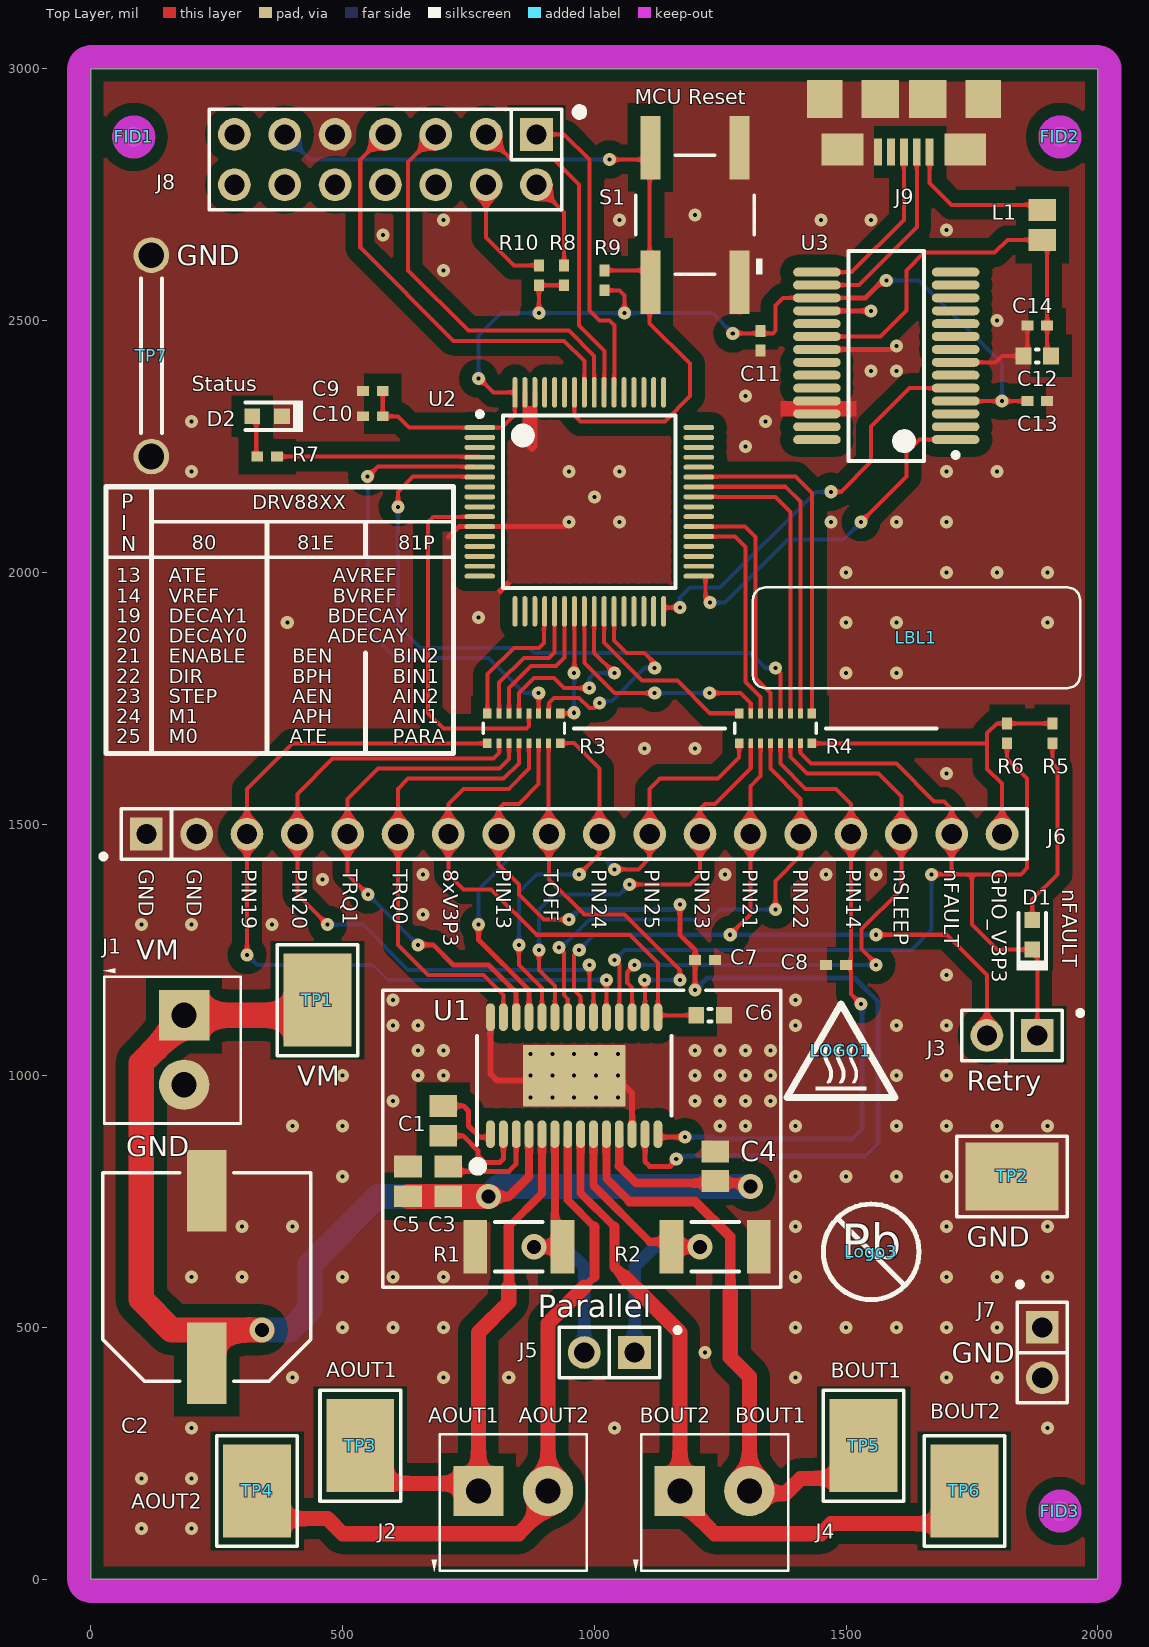
[diagram p0: Top Layer view]
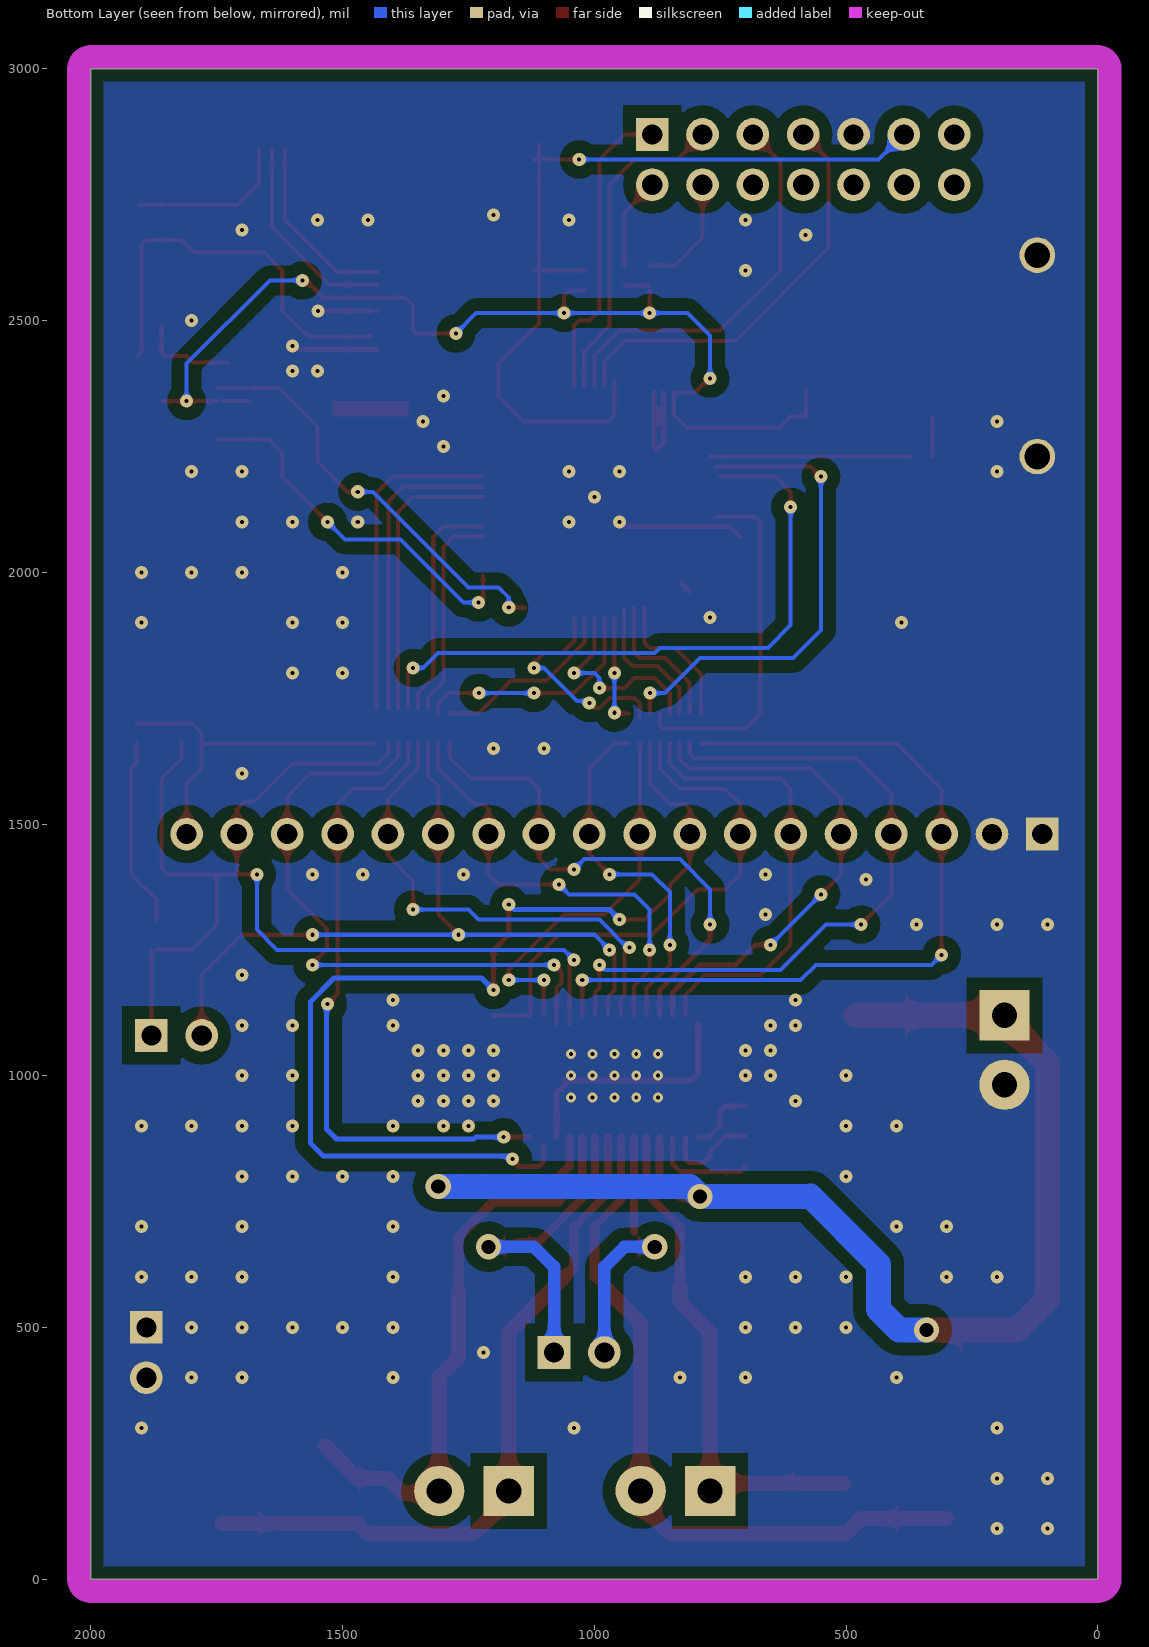
[diagram p1: Bottom Layer view, seen from below]
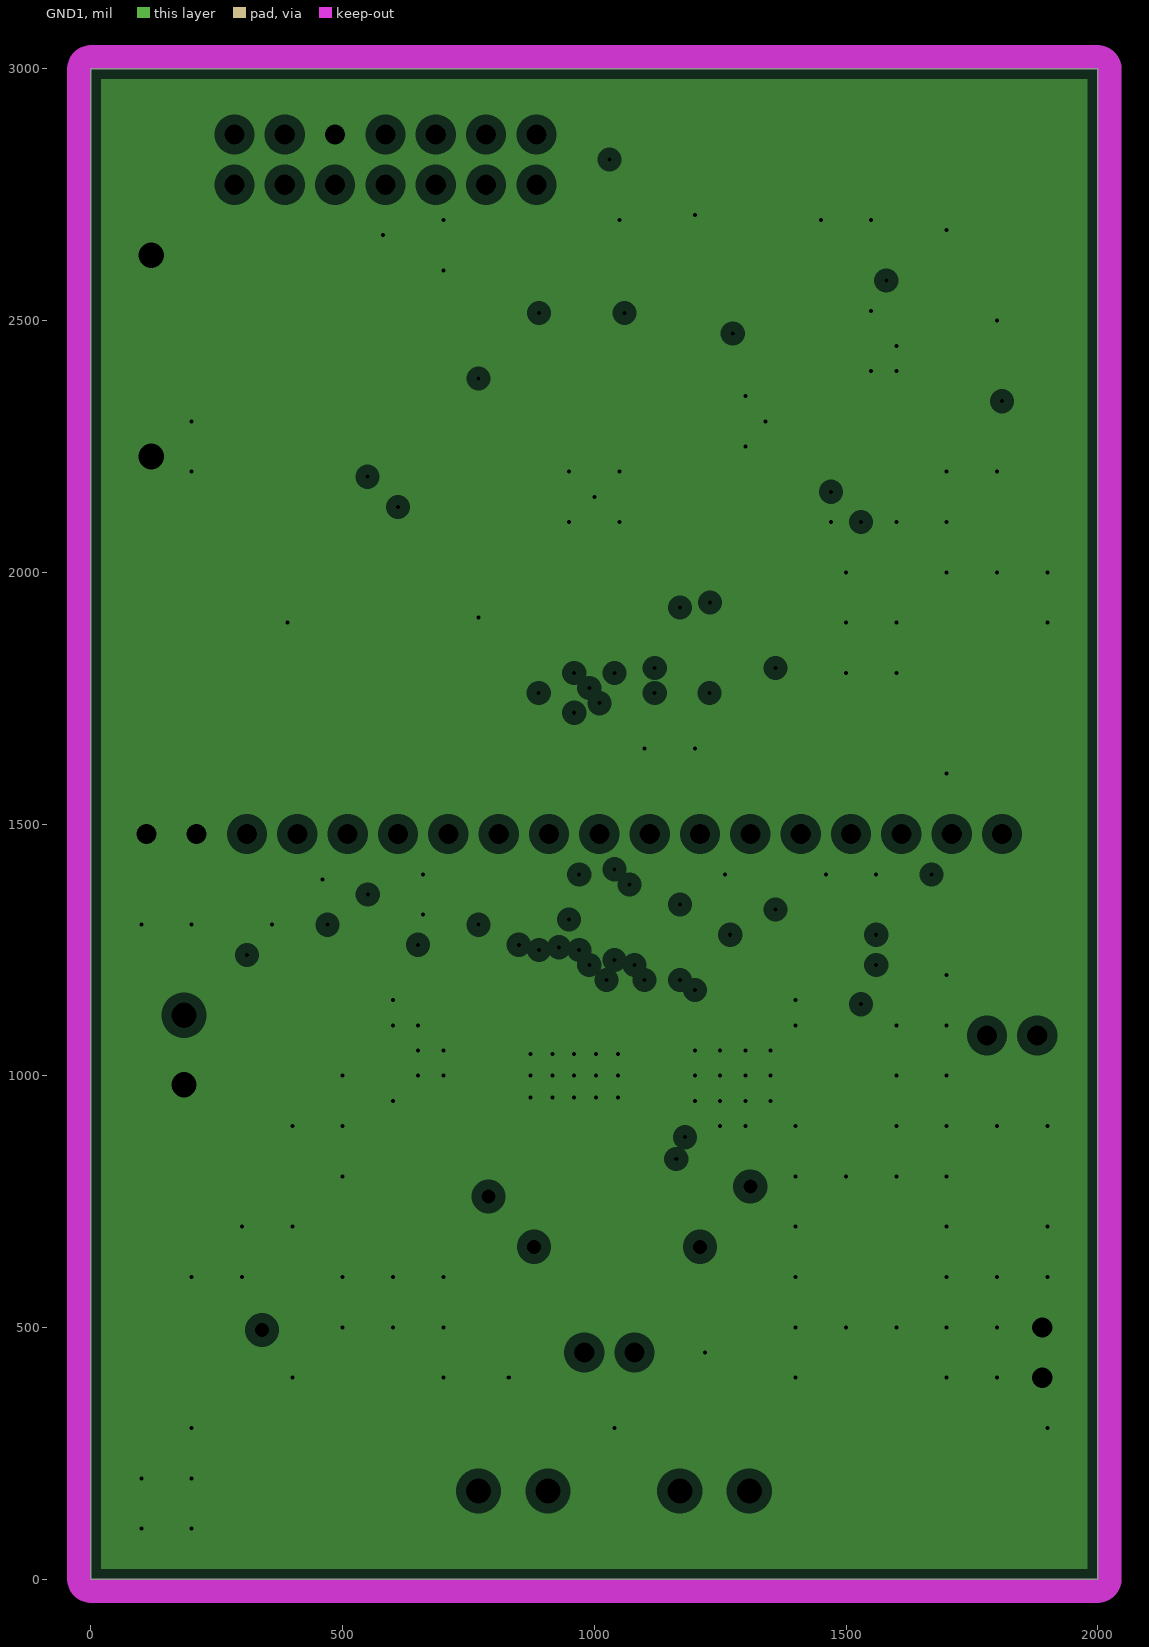
[diagram p2: GND1, clearances drawn from the general rule]
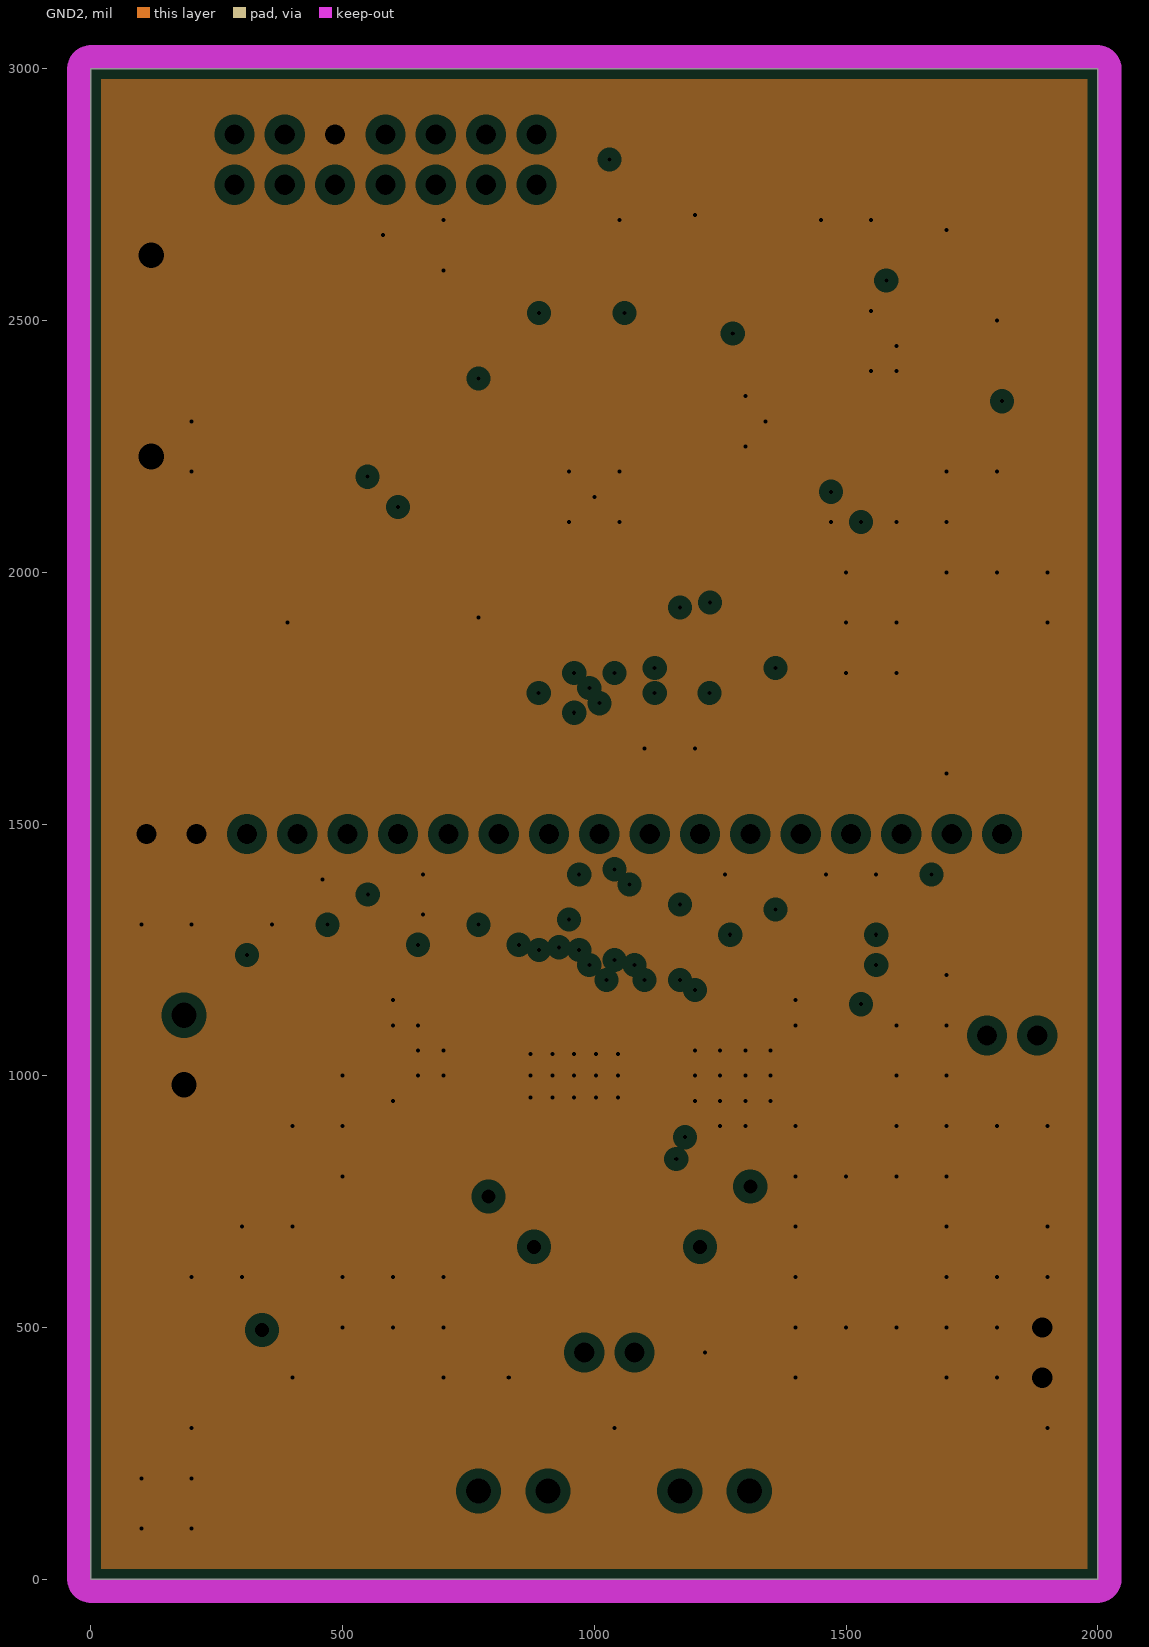
[diagram p3: GND2, clearances drawn from the general rule]
# Altium PCB MISC86176.PcbDoc (part 1 of 2)
Units mil, origin at the board's own origin, x right, y up, seen from the top; angles counter-clockwise.
Board outline 2000 x 3000 mil, 4 copper layers (Top Layer, GND1, GND2, Bottom Layer), stack 91.4 mil thick; 53 components, 60 nets, 274 pads, 201 vias.

## Layer stack, top to bottom
Top Layer: signal copper 2.1
Dielectric: core 59.2, FR-4, Dk 4.8
GND1: plane copper 1.4, net GND
Dielectric: prepreg 12.6, FR-4, Dk 4.8
GND2: plane copper 1.4, net GND
Dielectric: core 12.6, FR-4, Dk 4.8
Bottom Layer: signal copper 2.1

## Board outline
0,0 0,3000 2000,3000 2000,0

## Design rules (kind name [scope] priority, off if disabled: settings)
AcuteAngle [All] p1: minimum=4.50000000000000E+0001
Clearance Clearance_Keepouts [((IsTrack Or IsArc) And Not InPoly) And IsFree and IsKeepOut vs ((IsTrack Or IsArc) And Not InPoly) And IsFree and IsKeepOut] p1: gap=0
Clearance Clearance_BoardEdge_MountingHoles [OnCopper and InComponentClass('Mounting Holes') vs IsKeepOut] p2: gap=40
Clearance Clearance_BoardEdge_Poly [OnCopper and InPoly vs IsKeepOut] p3: gap=25
Clearance Clearance_BoardEdge [OnCopper and Not InComponentClass('Logo') and not InComponentClass('FiducialMark') and not InRegion(1000,500,4000,800) and Not IsKeepout vs IsKeepOut] p4: gap=20
Clearance Clearance_Poly [InPolygon] p5: gap=25
Clearance [All] p6: gap=7.87
ComponentClearance ComponentClearance_MountingHoles_FiducialMarks [InComponentClass('Mounting Holes') vs InComponentClass('FiducialMark')] p1: gap=50 collisioncheckmode=3 verticalgap=10 showdistances=FALSE
ComponentClearance ComponentClearance_Shunt [InComponentClass('Header') vs InComponentClass('Shunt')] p2: gap=0 collisioncheckmode=3 verticalgap=0 showdistances=FALSE
ComponentClearance ComponentClearance_Logo [InComponentClass('Logo')] p3: gap=50 collisioncheckmode=3 verticalgap=10 showdistances=FALSE
ComponentClearance ComponentClearance_ScrewToNut [(HasFootprint('NY PMS 440 0025 PH')) vs (HasFootprint('Keystone_1902C'))] p4: gap=5 collisioncheckmode=3 verticalgap=10 showdistances=FALSE
ComponentClearance ComponentClearance_MountingHoles [InComponentClass('Mounting Holes')] p5: gap=250 collisioncheckmode=3 verticalgap=100000 showdistances=FALSE
ComponentClearance ComponentClearance_SmallPassives [HasFootprint('0201*') or HasFootprint('0402*') or HasFootprint('0508') or HasFootprint('0603*') or HasFootprint('0612') or HasFootprint('0805*') or HasFootprint('0815*') or HasFootprint('0830*') or HasFootprint('1206*') or HasFootprint('1210*') or HasFootprint('1808*') or HasFootprint('1812*') or HasFootprint('1825*') or HasFootprint('2010*') or HasFootprint('2220*') or HasFootprint('2225*') or HasFootprint('2512*') or HasFootprint('2728*') or HasFootprint('3518*') vs HasFootprint('0201*') or HasFootprint('0402*') or HasFootprint('0508') or HasFootprint('0603*') or HasFootprint('0612') or HasFootprint('0805*') or HasFootprint('0815*') or HasFootprint('0830*') or HasFootprint('1206*') or HasFootprint('1210*') or HasFootprint('1808*') or HasFootprint('1812*') or HasFootprint('1825*') or HasFootprint('2010*') or HasFootprint('2220*') or HasFootprint('2225*') or HasFootprint('2512*') or HasFootprint('2728*') or HasFootprint('3518*')] p6: gap=20 collisioncheckmode=3 verticalgap=10 showdistances=FALSE
ComponentClearance ComponentClearance_THtoSMT [IsThruComponent vs IsSMTComponent] p7: gap=100 collisioncheckmode=3 verticalgap=30 showdistances=FALSE
ComponentClearance ComponentClearance_THtoTH [IsThruComponent vs IsThruComponent] p8: gap=118.11 collisioncheckmode=3 verticalgap=30 showdistances=FALSE
ComponentClearance [All] p9: gap=40 collisioncheckmode=3 verticalgap=10 showdistances=FALSE
DiffPairsRouting [All] p1: maxlimit=100 minlimit=10 mostfreqgap=10 maxuncoupledlength=1000
FabricationTestPointUsage TestPointUsage [All] p1: valid=2 allowmultiple=FALSE
FabricationTestpoint Testpoint [(IsPad And (OnTopLayer Or OnBottomLayer))] p1: side=3 testpointundercomponent=TRUE minsize=40 maxsize=100 preferedsize=60 minholesize=0 maxholesize=40 preferedholesize=32 testpointgrid=1 allowsidetop=TRUE allowsidebottom=TRUE usegrid=TRUE gridtolerance=0.01
FanoutControl Fanout_LCC [IsLCC] p1: bgadir=Out bgaviamode=Centered fanoutstyle=Auto fanoutdirection=Alternating viagrid=1 // Fanout_LCC (Default Rule)
FanoutControl Fanout_BGA [IsBGA] p2: bgadir=Out bgaviamode=Centered fanoutstyle=Auto fanoutdirection=Alternating viagrid=1 // Fanout_BGA (Default Rule)
FanoutControl Fanout_Default [All] p4: bgadir=Out bgaviamode=Centered fanoutstyle=Auto fanoutdirection=Alternating viagrid=1 // Fanout_Default (Default Rule)
FanoutControl Fanout_Small [(CompPinCount < 5)] p5: bgadir=Out bgaviamode=Centered fanoutstyle=Auto fanoutdirection=OutThenIn viagrid=1 // Fanout_Small (Default Rule)
HoleSize [All] p1: absolutevalues=TRUE maxlimit=251 minlimit=7.87 maxpercent=80.000 minpercent=20.000
MinimumAnnularRing MinimumAnnularRing_ThermalPadVias [IsVia and InAnyComponent] p1: minimumring=3.94
MinimumAnnularRing [All] p2: minimumring=5
MinimumSolderMaskSliver MinimumSolderMaskSliver_Logo [InComponentClass('Logo') vs InComponentClass('Logo')] p1: minsoldermaskwidth=0.7
MinimumSolderMaskSliver [All] p2: minsoldermaskwidth=3.94
PlaneClearance [All] p1: clearance=20
PlaneConnect [All] p1: planeconnectstyle=Relief reliefexpansion=10 reliefentries=4 reliefconductorwidth=10 reliefairgap=10
PolygonConnect PolygonConnect_2 [All vs IsNamedPolygon('Top Layer-GND')] p1: connectstyle=Direct reliefconductorwidth=10 reliefentries=4 polygonreliefangle="90 Angle"
PolygonConnect PolygonConnect_1 [All vs IsNamedPolygon('Bottom Layer-GND')] p2: connectstyle=Direct reliefconductorwidth=10 reliefentries=4 polygonreliefangle="90 Angle"
PolygonConnect [All] p3: connectstyle=Relief reliefconductorwidth=10 reliefentries=4 polygonreliefangle="90 Angle"
RoutingVias ThermalPadVias [IsVia and InAnyComponent] p1: holewidth=7.87 width=19.68 viastyle="Through Hole" minholewidth=7.87 minwidth=15.75 maxholewidth=12.99 maxwidth=23.62
RoutingVias [All] p2: holewidth=16 width=34 viastyle="Through Hole" minholewidth=7.87 minwidth=26 maxholewidth=40 maxwidth=65
SilkToSilkClearance SilkToSilkClearance_Pb-FreeLogo [(HasFootprint('Pb-Free_Overlay_Medium') OR HasFootprint('Pb-Free_Overlay_Small')) vs (HasFootprint('Pb-Free_Overlay_Medium') OR HasFootprint('Pb-Free_Overlay_Small'))] p1: silktosilkclearance=0
SilkToSilkClearance [All] p2: silktosilkclearance=3
SilkscreenOverComponentPads "Silk to Solder Mask Opening" [All] p1: minsilkscreentomaskgap=3
SolderMaskExpansion [All] p1: expansion=1.97
Width [All] p1: maxlimit=100 minlimit=6 preferedwidth=10 checkconnectedcopper=TRUE
14 further rules are at their usual default settings.

## Classes and differential pairs
component class Header: J3 J5 J6 J7 J8
component class MDBU004A_DRV888x: C1 C2 C3 C4 C5 C6 C7 C8 D1 J1 J2 J3 J4 J5 J6 J7 R1 R2 R3 R4 R5 R6 TP1 TP2 TP3 TP4 TP5 TP6 TP7 U1
component class MDBU004A_DRV888x_MSP430F2617: C9 C10 C11 C12 C13 C14 D2 J8 J9 L1 R7 R8 R9 R10 S1 U2 U3
component class Logo: Logo2
component class MDBU004A_Hardware: FID1 FID2 FID3 LBL1 LOGO1 Logo2 Logo3 Logo4 ZZ1 ZZ2 ZZ3 ZZ4 ZZ5
component class FiducialMark: FID1 FID2 FID3
component class AssemblyNote: ZZ1 ZZ2 ZZ3 ZZ4 ZZ5
component class Label: LBL1

## Components (designator, comment, footprint, x,y, rotation, side; value= is the part's Value field where it differs from the comment)
C1 "C0805C104K1RACTU" 0805L 700,910 r270 top
C2 "EEE-FK1J101P" SM_RADIAL_G 230,600 r90 top
C3 "C2012X7R1E474K" 0805L 710,790 r270 top
C4 "C0805C104K1RACTU" 0805L 1240,820 r270 top
C5 "C0805C104K1RACTU" 0805L 630,790 r270 top
C6 "C0603C474K9RACTU" 0603L 1230,1120 r0 top
C7 "GRM155R61A104KA01D" 0402L 1220,1230 r0 top
C8 "GRM155R61A104KA01D" 0402L 1480,1220 r180 top
C9 "GRM155R61A104KA01D" 0402L 560,2360 r180 top
C10 "GRM155R61A104KA01D" 0402L 560,2310 r180 top
C11 "GRM155R61A104KA01D" 0402L 1330,2460 r270 top
C12 "CGB3B1X5R1A475K055AC" 0603L 1880,2430 r180 top
C13 "GRM155R61A105KE15D" 0402L 1880,2340 r0 top
C14 "GRM155R61A104KA01D" 0402L 1880,2490 r180 top
D1 "LTST-C190CKT" LED_LTST-C190_Red 1870,1280 r270 top
D2 "LTST-C190GKT" LED_LTST-C190 350,2310 r0 top
FID1 "Fiducial" Fiducial10-20 85,2865 r90 top
FID2 "Fiducial" Fiducial10-20 1925,2865 r90 top
FID3 "Fiducial" Fiducial10-20 1925,135 r90 top
J1 "ED555/2DS" TERM_BLK_ED555-2DS 185,1120 r270 top
J2 "ED555/2DS" TERM_BLK_ED555-2DS 770,175 r0 top
J3 "90120-0122" CONN_90120-0122 1830,1080 r180 top
J4 "ED555/2DS" TERM_BLK_ED555-2DS 1170,175 r0 top
J5 "90120-0122" CONN_90120-0122 1030,450 r180 top
J6 "TSW-118-07-G-S" TSW-118-07-G-S 960,1480 r0 top
J7 "90120-0122" CONN_90120-0122 1890,450 r270 top
J8 "PEC07DAAN" CONN_PEC07DAAN 585,2820 r180 top
J9 "ZX62-B-5PA(11)" CONN_USB_micro_ZX62-B-5PA 1615,2835 r180 top
L1 "MMZ2012R300A" 0805L 1890,2690 r90 top
LBL1 "Size: 0.65\" x 0.20 \"" Label_650x200 1640,1870 r0 top
LOGO1 "CAUTION HOT SURFACE" IEC_HotSurface_Small 1490,1050 r0 top
Logo3 "Pb-Free Symbol" Pb-Free_Overlay_Medium 1550,650 r0 top
R1 "CSRN2010FKR250" 2010L 850,660 r0 top
R2 "CSRN2010FKR250" 2010L 1240,660 r180 top
R3 "EXB-2HV330JV" RESCAXS_EXB-2HV 860,1690 r0 top
R4 "EXB-2HV330JV" RESCAXS_EXB-2HV 1360,1690 r0 top
R5 "CRCW0402510RJNED" 0402L 1910,1680 r90 top
R6 "CRCW04024K99FKED" 0402L 1820,1680 r90 top
R7 "CRCW0402330RJNED" 0402L 350,2230 r0 top
R8 "ERJ-2GE0R00X" 0402L 940,2590 r90 top
R9 "CRCW04023K32FKED" 0402L 1020,2580 r270 top
R10 "ERJ-2GE0R00X" 0402L 890,2590 r90 top
S1 "EVQP1D05M" SW_EVQxxx05M 1200,2710 r180 top
TP1 "5016" Testpoint_Keystone_Compact 450,1150 r90 top
TP2 "5016" Testpoint_Keystone_Compact 1830,800 r180 top
TP3 "5016" Testpoint_Keystone_Compact 535,265 r90 top
TP4 "5016" Testpoint_Keystone_Compact 330,175 r90 top
TP5 "5016" Testpoint_Keystone_Compact 1535,265 r90 top
TP6 "5016" Testpoint_Keystone_Compact 1735,175 r90 top
TP7 "D3082-05" Harwin_D3082-05 120,2430 r270 top
U1 "DRV8880PWPR" PWP0028C_N 960,1000 r90 top
U2 "MSP430F2617TPM" PM0064A_L 990,2140 r0 top
U3 "FT232RL" SSOP28_M 1580,2430 r180 top

## Footprints (in the part's own frame and the unit in brackets; to place one, negate y for a bottom-side part, rotate by r counter-clockwise, add the part's x,y. Pads: shape width x height; smd on the part's side, far side on the other; paste and mask are expansions set on the pad)
0402L [mm] "0402 from SM-752 data"
  rect 0.6x0.5 smd: 1(-0.5,0) 2(0.5,0)
  body extent -0.55,-0.3 0.55,0.3, height 0.6
0603L [mm] "0603 from SM-752 data"
  rect 0.8x0.85 smd: 1(-0.7,0) 2(0.7,0)
  silkscreen extent -0.07,-0.33 0.07,0.33, body extent -0.87,-0.47 0.87,0.47, height 0.85
0805L [mm] "0805 from SM-752 data"
  rect 1.1x1.4 smd: 1(-0.75,0) 2(0.75,0)
  body extent -1.1,-0.72 1.1,0.72, height 1.1
2010L [mm]
  rect 1.2x2.7 smd: 1(-2.2,0) 2(2.2,0)
  silkscreen extent -1.2,-1.25 1.2,1.25, body extent -2.73,-1.45 2.73,1.45, height 1.66
CONN_90120-0122 [mm] "Molex"
  rect 1.65x1.65 hole 1.016 mask+0: 1(-1.27,0)
  round 1.65 hole 1.016 mask+0: 2(1.27,0)
  silkscreen extent -3.57,-1.27 2.54,1.27, body extent -2.54,-1.27 2.54,1.27, height 9.29
CONN_PEC07DAAN [mm] "SULLINS"
  rect 1.65x1.65 hole 1.016 mask+0: 1(-7.62,-1.27)
  round 1.65 hole 1.016 mask+0: 2(-7.62,1.27) 3(-5.08,-1.27) 4(-5.08,1.27) 5(-2.54,-1.27) 6(-2.54,1.27) 7(0,-1.27) 8(0,1.27) 9(2.54,-1.27) 10(2.54,1.27) 11(5.08,-1.27) 12(5.08,1.27) 13(7.62,-1.27) 14(7.62,1.27)
  silkscreen extent -9.99,-2.6 8.89,2.54, body extent -8.95,-2.6 8.95,2.6, height 11.43
CONN_USB_micro_ZX62-B-5PA [mm] "Hirose"
  rect 0.4x1.35 smd: 1(-1.3,0) 2(-0.65,0) 3(0,0) 4(0.65,0) 5(1.3,0)
  rect 1.9x1.9 smd: 6(-1.2,-2.675) 7(1.2,-2.675)
  rect 1.8x1.9 smd: 8(-4,-2.675) 9(4,-2.675)
  rect 2.1x1.6 smd: 10(-3.1,-0.125) 11(3.1,-0.125)
  body extent -3.75,-5.32 3.75,0.18, height 2.55
Fiducial10-20 [mm]
  round 1 smd mask+0.5: 1(0,0)
  Top Layer keep-out circle w1.178: c0,0 r0.5
Harwin_D3082-05 [mm] "Shorting Plug, 10.16mm spacing, TH"
  round 1.8 hole 1.3: 1(-5.08,0) 2(5.08,0)
  silkscreen extent -3.9,-0.53 3.9,0.53, body extent -5.6,-0.52 5.61,0.52, height 6.63
IEC_HotSurface_Small [mil]
  silkscreen extent -107,-93 107,92
Label_650x200 [mil] "Thermal Transfer Label"
  round 1 on Mech13: 0(0,0)
  silkscreen extent -325,-100 325,100, body extent -326,-101 326,101, height 1
LED_LTST-C190 [mm] "Lite-On"
  rect 0.8x0.8 smd: 1(-0.75,0) 2(0.75,0)
  silkscreen extent -1.1,-0.8 1.8,0.8, body extent -0.85,-0.45 0.85,0.45, height 0.9
LED_LTST-C190_Red [mm] "Lite-On"
  rect 0.8x0.8 smd: 1(-0.75,0) 2(0.75,0)
  silkscreen extent -1.1,-0.8 1.8,0.8, body extent -0.85,-0.45 0.85,0.45, height 0.9
Pb-Free_Overlay_Medium [mil]
  silkscreen extent -95,-95 95,95
PM0064A_L [mm] "Thin QFP, 64-Leads, Body 10x10mm, Pitch 0.5mm, IPC High Density"
  oval 1.55x0.25 smd: 1(-5.525,3.75) 2(-5.525,3.25) 3(-5.525,2.75) 4(-5.525,2.25) 5(-5.525,1.75) 6(-5.525,1.25) 7(-5.525,0.75) 8(-5.525,0.25) 9(-5.525,-0.25) 10(-5.525,-0.75) 11(-5.525,-1.25) 12(-5.525,-1.75) 13(-5.525,-2.25) 14(-5.525,-2.75) 15(-5.525,-3.25) 16(-5.525,-3.75) 33(5.525,-3.75) 34(5.525,-3.25) 35(5.525,-2.75) 36(5.525,-2.25) 37(5.525,-1.75) 38(5.525,-1.25) 39(5.525,-0.75) 40(5.525,-0.25) 41(5.525,0.25) 42(5.525,0.75) 43(5.525,1.25) 44(5.525,1.75) 45(5.525,2.25) 46(5.525,2.75) 47(5.525,3.25) 48(5.525,3.75)
  oval 0.25x1.55 smd: 17(-3.75,-5.525) 18(-3.25,-5.525) 19(-2.75,-5.525) 20(-2.25,-5.525) 21(-1.75,-5.525) 22(-1.25,-5.525) 23(-0.75,-5.525) 24(-0.25,-5.525) 25(0.25,-5.525) 26(0.75,-5.525) 27(1.25,-5.525) 28(1.75,-5.525) 29(2.25,-5.525) 30(2.75,-5.525) 31(3.25,-5.525) 32(3.75,-5.525) 49(3.75,5.525) 50(3.25,5.525) 51(2.75,5.525) 52(2.25,5.525) 53(1.75,5.525) 54(1.25,5.525) 55(0.75,5.525) 56(0.25,5.525) 57(-0.25,5.525) 58(-0.75,5.525) 59(-1.25,5.525) 60(-1.75,5.525) 61(-2.25,5.525) 62(-2.75,5.525) 63(-3.25,5.525) 64(-3.75,5.525)
  silkscreen extent -5.65,-4.35 4.35,4.55, body extent -5,-5 5,5, height 1.61
PWP0028C_N [mm] "TSOP, 28-Leads, Body 9.7x4.4mm, Pitch 0.65mm, Exposed Pad, IPC Medium Density"
  rrect100% 1.4x0.45 smd: 1(-2.95,4.225) 2(-2.95,3.575) 3(-2.95,2.925) 4(-2.95,2.275) 5(-2.95,1.625) 6(-2.95,0.975) 7(-2.95,0.325) 8(-2.95,-0.325) 9(-2.95,-0.975) 10(-2.95,-1.625) 11(-2.95,-2.275) 12(-2.95,-2.925) 13(-2.95,-3.575) 14(-2.95,-4.225) 15(2.95,-4.225) 16(2.95,-3.575) 17(2.95,-2.925) 18(2.95,-2.275) 19(2.95,-1.625) 20(2.95,-0.975) 21(2.95,-0.325) 22(2.95,0.325) 23(2.95,0.975) 24(2.95,1.625) 25(2.95,2.275) 26(2.95,2.925) 27(2.95,3.575) 28(2.95,4.225)
  rrect3% 3.1x5.18 smd: 29(0,0)
  silkscreen extent -3.5,-4.9 2,4.9, body extent -3.21,-4.85 3.21,4.85, height 0.98
RESCAXS_EXB-2HV [mm] "Panasonic Resistor Array"
  rect 0.425x0.5 smd mask+0.07: 1(-1.837,-0.75) 8(1.837,-0.75) 9(1.837,0.75) 16(-1.837,0.75)
  rect 0.25x0.5 smd mask+0.07: 2(-1.25,-0.75) 3(-0.75,-0.75) 4(-0.25,-0.75) 5(0.25,-0.75) 6(0.75,-0.75) 7(1.25,-0.75) 10(1.25,0.75) 11(0.75,0.75) 12(0.25,0.75) 13(-0.25,0.75) 14(-0.75,0.75) 15(-1.25,0.75)
  silkscreen extent -2.05,-0.25 2.05,0.25, body extent -1.95,-0.8 1.95,0.8, height 0.55
SM_RADIAL_G [mm] "10 x 10.2mm:  Panasonic G"
  rect 4.1x2 smd: 1(-4.35,0) 2(4.35,0)
  silkscreen extent -5.25,-5.25 5.25,5.25, body extent -5.26,-5.26 5.26,5.26, height 10.5
SSOP28_M [mm] "SOP, 28-Leads, Body 10.2x5.3mm, Pitch 0.65mm, IPC Low Density"
  oval 2.4x0.45 smd: 1(-3.5,4.225) 2(-3.5,3.575) 3(-3.5,2.925) 4(-3.5,2.275) 5(-3.5,1.625) 6(-3.5,0.975) 7(-3.5,0.325) 8(-3.5,-0.325) 9(-3.5,-0.975) 10(-3.5,-1.625) 11(-3.5,-2.275) 12(-3.5,-2.925) 13(-3.5,-3.575) 14(-3.5,-4.225) 15(3.5,-4.225) 16(3.5,-3.575) 17(3.5,-2.925) 18(3.5,-2.275) 19(3.5,-1.625) 20(3.5,-0.975) 21(3.5,-0.325) 22(3.5,0.325) 23(3.5,0.975) 24(3.5,1.625) 25(3.5,2.275) 26(3.5,2.925) 27(3.5,3.575) 28(3.5,4.225)
  silkscreen extent -3.63,-5.3 1.9,5.3, body extent -2.7,-5.3 2.7,5.3, height 2
SW_EVQxxx05M [mm] "Panasonic EVQP0/EVQP1/EVQ9P 6mm Square Long Travel Light Touch Switch"
  rect 1x3.2 smd: 1(-2.25,3.4) 2(-2.25,-3.4) 3(2.25,-3.4) 4(2.25,3.4)
  silkscreen extent -3.4,-3 3,3, body extent -3,-3 3,3, height 5
TERM_BLK_ED555-2DS [mil]
  rect 100x100 hole 50: 1(0,0)
  round 100 hole 50: 2(138,0)
  silkscreen extent -93,-161 215,113, body extent -69,-150 207,106, height 323
Testpoint_Keystone_Compact [mil] "Compact SMT test point"
  rect 185x135 smd: 1(0,0)
  silkscreen extent -110,-80 110,80, body extent -75,-56 75,56, height 91
TSW-118-07-G-S [mm] "Samtec 100mil, 1x18, 230 mil above insulator"
  rect 1.65x1.65 hole 1.016 mask+0: 1(-21.59,0)
  round 1.65 hole 1.016 mask+0: 2(-19.05,0) 3(-16.51,0) 4(-13.97,0) 5(-11.43,0) 6(-8.89,0) 7(-6.35,0) 8(-3.81,0) 9(-1.27,0) 10(1.27,0) 11(3.81,0) 12(6.35,0) 13(8.89,0) 14(11.43,0) 15(13.97,0) 16(16.51,0) 17(19.05,0) 18(21.59,0)
  silkscreen extent -23.88,-1.27 22.86,1.27, body extent -22.86,-1.27 22.86,1.27, height 8.38

## Part data
C1 C4 C5: "CAP, CERM, 0.1 μF, 100 V, +/- 10%, X7R, 0805"
C2: "CAP, AL, 100 μF, 63 V, +/- 20%, 0.35 ohm, SMD"
C3: "CAP, CERM, 0.47 μF, 25 V, +/- 10%, X7R, 0805"
C6: "CAP, CERM, 0.47 μF, 6.3 V, +/- 10%, X7R, 0603"
C7 C8 C9 C10 C11 C14: "CAP, CERM, 0.1 μF, 10 V, +/- 10%, X5R, 0402"
C12: "CAP, CERM, 4.7 μF, 10 V, +/- 10%, X5R, 0603"
C13: "CAP, CERM, 1 μF, 10 V, +/- 10%, X5R, 0402"
D1: "LED, Red, SMD"
D2: "LED, Green, SMD"
FID1 FID2 FID3: "Fiducial mark.  There is nothing to buy or mount."
J1 J2 J4: "Terminal Block, 6A, 3.5mm Pitch, 2-Pos, TH"
J3 J5 J7: "Header, 100mil, 2x1, Tin, TH"
J6: "Header, 100mil, 18x1, Gold, TH"
J8: "Header, 100mil, 7x2, Tin, TH"
J9: "Connector, Receptacle, Micro-USB Type B, R/A, Bottom Mount SMT"
L1: "Ferrite Bead, 30 ohm @ 100 MHz, 1.5 A, 0805"
LBL1: library part THT-14-423-10, "Thermal Transfer Printable Labels, 0.650\" W x 0.200\" H - 10,000 per roll"
LOGO1: library part IEC_HotSurface, "IEC 61010-1 Hot Surface Warning"
Logo3: library part Pb-Free
R1 R2: "RES, 0.25, 1%, 1 W, 2010"
R3 R4: "RES, 33, 5%, 0.0625 W, Resistor Array - 8x1"
R5: "RES, 510, 5%, 0.063 W, 0402"
R6: "RES, 4.99 k, 1%, 0.063 W, 0402"
R7: "RES, 330, 5%, 0.063 W, 0402"
R8 R10: "RES, 0, 5%, 0.063 W, 0402"
R9: "RES, 3.32 k, 1%, 0.063 W, 0402"
S1: "Switch, Tactile, SPST-NO, 0.05A, 12V, SMT"
TP1 TP2 TP3 TP4 TP5 TP6: "Test Point, Compact, SMT"
TP7: "1mm Uninsulated Shorting Plug, 10.16mm spacing, TH"
U1: "2-A 45-V 1/16-Microstep Stepper Motor Driver With AutoTune, PWP0028C"
U2: "16 MHz Mixed Signal Microcontroller with 92 KB Flash, 8192 B SRAM and 48 GPIOs, -40 to 105 degC, 64-pin QFP (PM), Green (RoHS & no Sb/Br)"
U3: "USB to Serial UART, SSOP28"

## Via types
v1: diameter 26, hole 8, Top Layer to Bottom Layer, tented both sides, 180 vias
v2: diameter 19.68, hole 7.87, Top Layer to Bottom Layer, 15 vias
v3: diameter 50, hole 28, Top Layer to Bottom Layer, tented both sides, 5 vias
v4: diameter 26, hole 8, Top Layer to Bottom Layer, tented top, 1 vias

## Nets (pads, with @x,y where several pads share a name; then routed paths per layer and width w, separated by ;. In a path a pad name is that pad's centre, name@x,y a point inside that pad or via, vN(x,y) a via of type N, cw(c..) or ccw(c..) an arc to the next point about the centre after c; other vN are vias at no path point)
8XV3P3: C6.1 J6.7 R3.5 U1.15 | length 1048.5
  Top Layer w8: R3.5@869.84,1660.47 869.84,1609.84 830,1570 740,1570 710,1540 J6.7@710,1480 710,1400 740,1370 795,1370 885,1280 1070,1280 1126.34,1223.66 1126.34,1120 C6.1@1202.44,1120
AISEN: J5.2 R1.2 U1.6 | length 551.6
  Top Layer w16: R1.2@921.61,690 U1.6@921.61,877.8
  Top Layer w25: v3@869.68,660 v3(880,660) R1.2@936.61,660
  Bottom Layer w25: v3@869.68,660 v3(880,660) 940,660 980,620 J5.2@980,450
AOUT1: J2.1 TP3.1 U1.5 | length 1001.3
  Top Layer w16: 830,700 896.02,766.02 U1.5@896.02,877.8
  Top Layer w20: 830,580 830,700
  Top Layer w30: TP3.1@503.69,190.08 514.98,190.08 534.98,190.07 J2.1@750,190 ; J2.1@770,175 770,490 830,550 830,580
AOUT2: J2.2 TP4.1 U1.7 | length 1434.2
  Top Layer w16: U1.7@947.2,877.8 947.2,752.8 1000,700 ; 980,580 1000,600
  Top Layer w20: 1000,600 1000,700
  Top Layer w30: TP4.1@300,120 470,120 500,90 850,90 908,148 J2.2@908,175 908,508 980,580
BISEN: J5.1 R2.2 U1.9 | length 669.4
  Top Layer w16: U1.9@998.39,877.8 998.39,781.61 1110,670 R2.2@1152.2,670
  Top Layer w25: R2.2@1153.39,660 v3(1210,660)
  Bottom Layer w25: J5.1@1080,450 1080,620 1120,660 v3(1210,660)
BOUT1: J4.2 TP5.1 U1.10 | length 1145
  Top Layer w16: U1.10@1023.98,877.8 1023.98,796.02 1070,750
  Top Layer w20: 1070,750 1200,750 1270,680 1270,570
  Top Layer w30: 1270,570 1270,440 1308,402 J4.2@1308,175 ; J4.2@1328,175 1333,170 1380,170 1410,200 1470,200 TP5.1@1535,265
BOUT2: J4.1 TP6.1 U1.8 | length 1407.4
  Top Layer w16: U1.8@972.8,877.8 972.8,767.2 1040,700
  Top Layer w20: 1040,700 1040,620 1060,600
  Top Layer w30: 1060,600 1170,490 J4.1@1170,175 1170,158.9 1238.9,90 1450,90 1470,110 TP6.1@1740,110
DM: J9.2 U3.16 | length 411.6
  Top Layer w8: U3.16@1430.9,2570.8 1525.8,2570.8 1640.59,2685.59 J9.2@1640.59,2835 J9.2@1640.59,2840
DP: J9.3 U3.15 | length 367
  Top Layer w8: U3.15@1430.9,2596.4 1511.4,2596.4 1615,2700 J9.3@1615,2835 J9.3@1615,2840